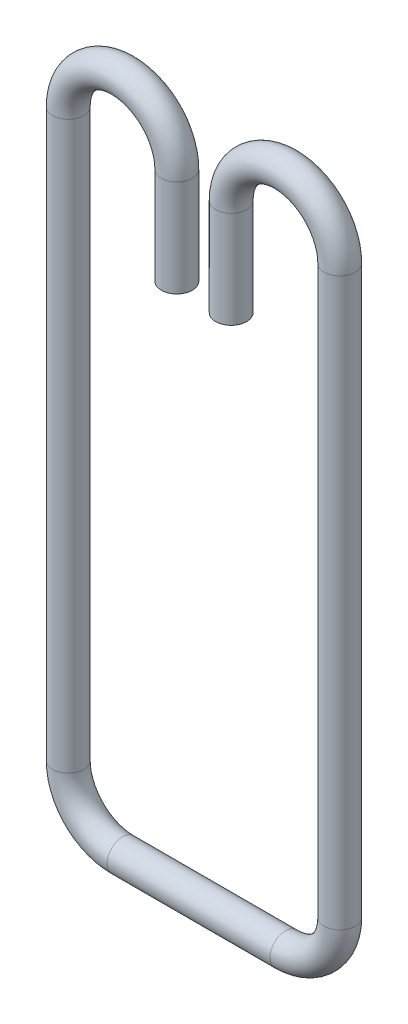
SolidWorks part; units mm, degrees
material "A3"
ref_plane "前视基准面" through (0, 0, 0) normal (0, 0, 1) x (1, 0, 0)
ref_plane "上视基准面" through (0, 0, 0) normal (0, 1, 0) x (1, 0, 0)
ref_plane "右视基准面" through (0, 0, 0) normal (1, 0, 0) x (0, 0, -1)
sketch "草图1" plane through (0, 0, 0) normal (0, 0, 1) x (1, 0, 0)
  line L0 (42, 0) -> (-42, 0)
  line L1 (-70, 28) -> (-70, 320)
  line L2 (-70, 320) -> (-14, 320) construction
  line L3 (-14, 320) -> (-14, 270)
  line L4 (0, 0) -> (0, 89.6721) construction
  line L5 (70, 320) -> (14, 320) construction
  line L6 (14, 320) -> (14, 270)
  line L7 (70, 28) -> (70, 320)
  arc A0 (-14, 320) -> (-70, 320) centre (-42, 320) ccw
  arc A1 (-42, 0) -> (-70, 28) centre (-42, 28) cw
  arc A2 (42, 0) -> (70, 28) centre (42, 28) ccw
  arc A3 (14, 320) -> (70, 320) centre (42, 320) cw
  dimension "D1" = 70
  dimension "D2" = 28
  dimension "D5" = 28
  dimension "D3" = 50
  dimension "D4" = 320
sweep "扫描1" add path "草图1" circular profile diameter 16 parameters "D3"=16
